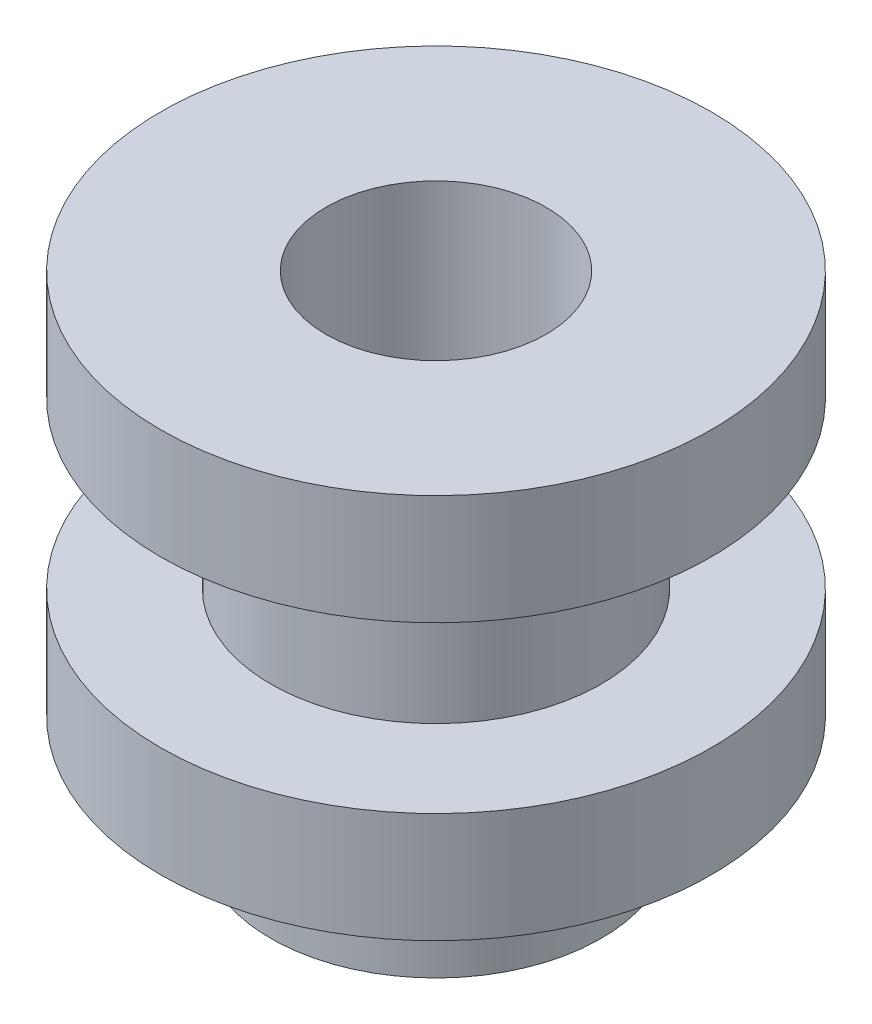
from build123d import *

# Parameters (mm, degrees)
SKETCH1_R           = 5
BOSS_EXTRUDE1_DEPTH = 9
SKETCH3_W           = 2
SKETCH3_H           = 3
SKETCH3_H_2         = 2
SKETCH4_R           = 2
CUT_EXTRUDE1_DEPTH  = 12.445523142


with BuildPart() as part:
    # Sketch1 → Boss-Extrude1 (new body)
    with BuildSketch(Plane(origin=(0, 0, 0), x_dir=(1, 0, 0), z_dir=(0, 1, 0))):
        with Locations(Location((0, 0, 0), (0, 0, 270))):
            Circle(SKETCH1_R)
    extrude(amount=BOSS_EXTRUDE1_DEPTH)

    # Sketch3 → Cut-Revolve1 (revolve, cut)
    with BuildSketch(Plane.XY, mode=Mode.PRIVATE) as cut_revolve1_sk:
        with Locations((4, 5.5)):
            Rectangle(SKETCH3_W, SKETCH3_H)
        with Locations((4, 1)):
            Rectangle(SKETCH3_W, SKETCH3_H_2)
    revolve(cut_revolve1_sk.sketch.rotate(Axis((0, 0, 0), (0, 1, 0)), 90), axis=Axis((0, 0, 0), (0, 1, 0)), mode=Mode.SUBTRACT)

    # Sketch4 → Cut-Extrude1 (cut, through all)
    with BuildSketch(Plane(origin=(0, 9, 0), x_dir=(1, 0, 0), z_dir=(0, 1, 0))):
        with Locations(Location((0, 0, 0), (0, 0, 270))):
            Circle(SKETCH4_R)
    extrude(amount=-CUT_EXTRUDE1_DEPTH, mode=Mode.SUBTRACT)


solid = part.part
